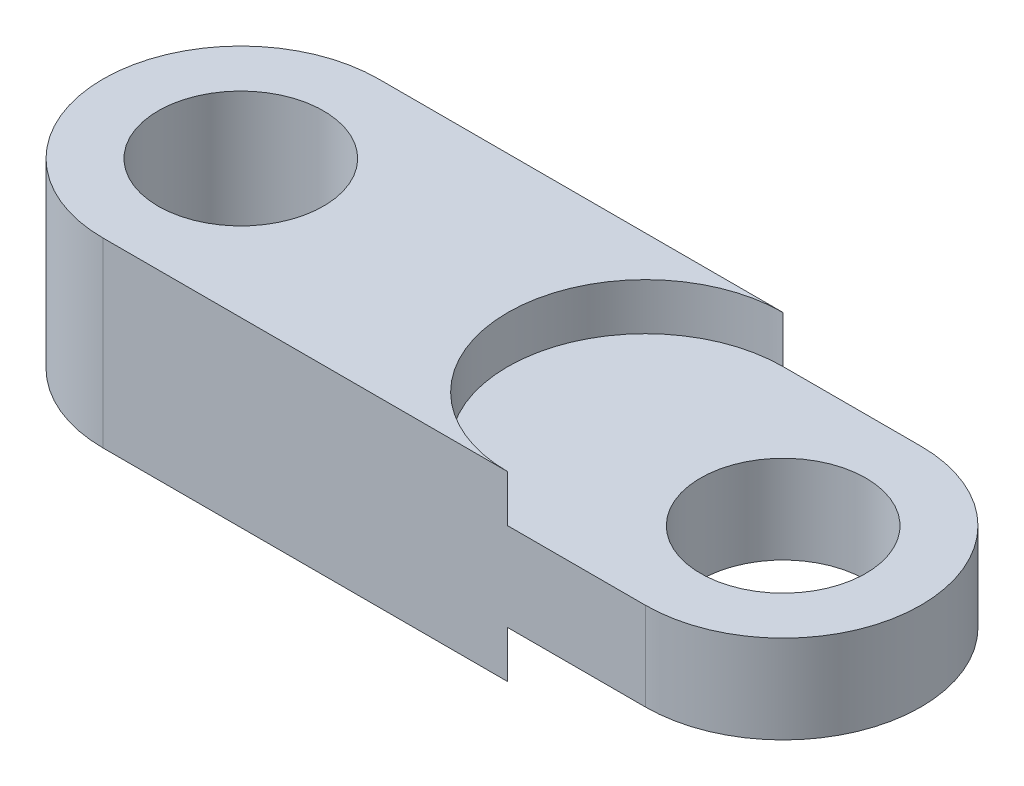
SolidWorks part; units mm, degrees
ref_plane "Front Plane" through (0, 0, 0) normal (0, 0, 1) x (1, 0, 0)
ref_plane "Top Plane" through (0, 0, 0) normal (0, 1, 0) x (1, 0, 0)
ref_plane "Right Plane" through (0, 0, 0) normal (1, 0, 0) x (0, 0, -1)
sketch "Sketch2" plane through (0, 0, 0) normal (0, 1, 0) x (1, 0, 0)
  line L0 (0, 0) -> (25, 0) construction
  line L1 (0, 6.35) -> (25, 6.35)
  line L2 (0, -6.35) -> (25, -6.35)
  arc A0 (0, 6.35) -> (0, -6.35) centre (0, 0) ccw
  arc A1 (25, -6.35) -> (25, 6.35) centre (25, 0) ccw
  circle A2 centre (0, 0) radius 3.81
  circle A3 centre (25, 0) radius 3.81
  point P3 (12.5, 0)
  dimension "D1" = 6.35
  dimension "D3" = 7.62
  dimension "D4" = 7.62
  dimension "D2" = 25
extrude "Boss-Extrude1" add sketch "Sketch2" along normal blind 8.382
sketch "Sketch3" plane through (0, 0, 6.35) normal (0, 0, 1) x (1, 0, 0)
  line L0 (18.65, 8.382) -> (18.65, 6.223)
  line L1 (0, 8.382) -> (25, 8.382) construction
  line L2 (18.65, 6.223) -> (51.556, 6.223)
  line L3 (18.65, 2.159) -> (18.65, 0)
  line L4 (0, 0) -> (25, 0) construction
  line L5 (18.65, 2.159) -> (52.1425, 2.159)
  line L6 (0, 4.191) -> (39.3856, 4.191) construction
  line L7 (0, 8.382) -> (0, 0) construction
  line L8 (18.65, 6.223) -> (18.65, 2.159) construction
  line L9 (25, 8.382) -> (25, 0) construction
  line L10 (12.4272, 8.382) -> (49.8313, 8.382)
  line L11 (49.8313, 8.382) -> (51.556, 6.223)
  line L12 (18.65, 0) -> (54.0397, 0)
  line L13 (54.0397, 0) -> (52.1425, 2.159)
  line M1 (0, 0) -> (25, 0)
  line M2 (25, 0) -> (25, 8.382)
  line M3 (25, 8.382) -> (0, 8.382)
  dimension "D1" = 2.032
  dimension "D2" = 2.032
  dimension "D3" = 6.35
extrude "Cut-Extrude3" cut sketch "Sketch3" against normal through all contours L12 L13 L5 M2 | L5 L3 M1 M2 | L11 L10 L2 M2 | L0 L2 M2 M3
sketch "Sketch4" plane through (0, 0, 0) normal (0, -1, 0) x (1, 0, 0)
  line L0 (18.65, -6.35) -> (18.65, 6.35) construction
  line L1 (18.65, -6.35) -> (0, -6.35) construction
  circle A0 centre (18.65, 0) radius 6.35
extrude "Cut-Extrude5" cut sketch "Sketch4" against normal up to surface (2.159 mm away) up to face at (25, 2.159, -3.81)
sketch "Sketch5" plane through (0, 8.382, 0) normal (0, 1, 0) x (1, 0, 0)
  line L0 (18.65, 6.35) -> (18.65, -6.35) construction
  circle A0 centre (18.65, 0) radius 6.35
extrude "Cut-Extrude6" cut sketch "Sketch5" against normal up to surface (2.159 mm away) up to face at (25, 6.223, -3.81)
scale "Scale1" bodies to scale 104 scale about origin uniform scaling yes scale factor 2
